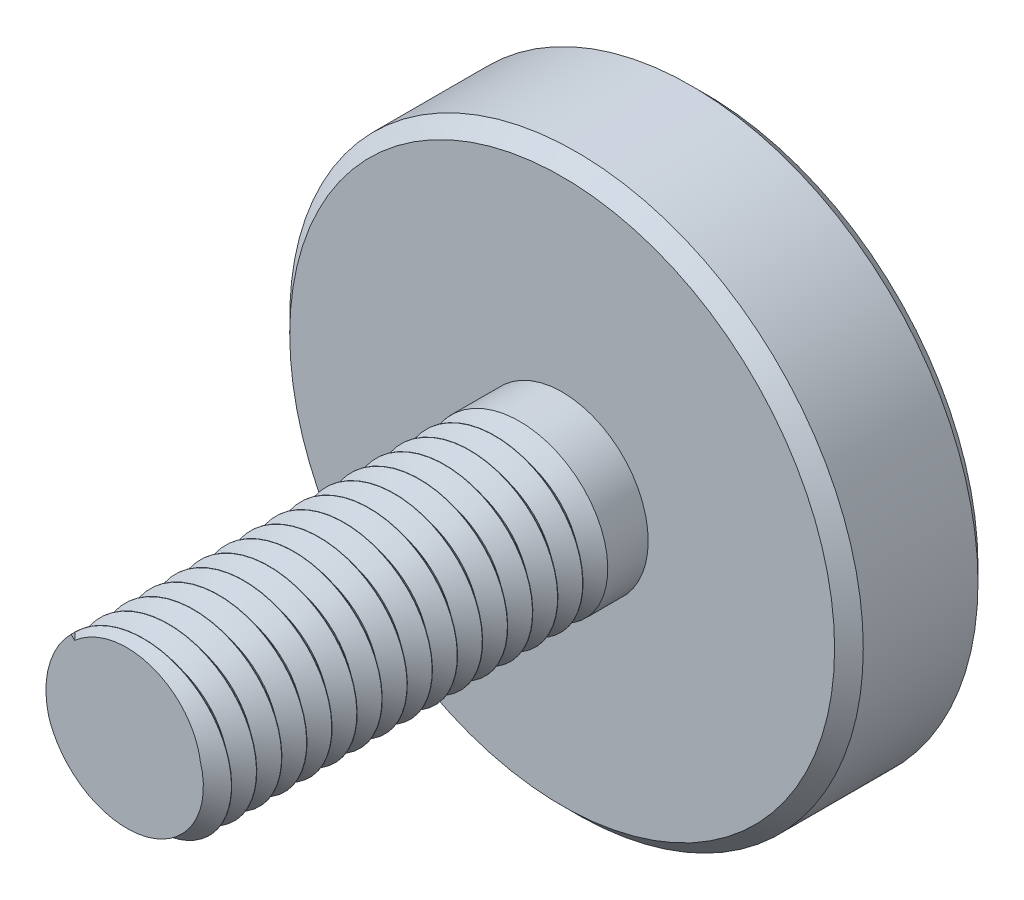
from build123d import *

# Parameters (mm, degrees)
SKETCH_1_R          = 20
EXTRUDE_1_DEPTH     = 10
SKETCH_2_R          = 6
EXTRUDE_3_DEPTH     = 30
SWEEP_1_PITCH       = 1.75
SWEEP_1_HEIGHT      = 28
SWEEP_1_RADIUS      = 6
SWEEP_1_START_ANGLE = 45
CHAMFER_1_SIZE      = 1


with BuildPart() as part:
    # 草图1 → 凸台-拉伸1 (new body)
    with BuildSketch(Plane.XY):
        Circle(SKETCH_1_R)
    extrude(amount=EXTRUDE_1_DEPTH)

    # 草图2 → 凸台-拉伸3 (add)
    with BuildSketch(Plane.XY.offset(10)):
        Circle(SKETCH_2_R)
    extrude(amount=EXTRUDE_3_DEPTH)

    # 切除-扫描1: sweep along a helix
    with BuildLine() as sweep_1_path:
        add(Helix(SWEEP_1_PITCH, SWEEP_1_HEIGHT, SWEEP_1_RADIUS, center=(0, 0, 40), direction=(0, 0, -1), mode=Mode.PRIVATE).rotate(Axis((0, 0, 40), (0, 0, -1)), SWEEP_1_START_ANGLE))
    # 草图5 → 切除-扫描1 (sweep, cut)
    with BuildSketch(Plane(origin=(0, 0, 0), x_dir=(0, 0, -1), z_dir=(1, 0, 0))):
        Polygon((-39.598251524, 6.141374382), (-37.652469247, 6.141374382), (-38.625360385, 4.883734618), align=None)
    sweep(path=sweep_1_path.line, is_frenet=True, mode=Mode.SUBTRACT)

    # 倒角1
    chamfer_1_edges = [part.edges().sort_by_distance(p)[0] for p in [
        (-20, 0, 0),
        (-20, 0, 10),
    ]]
    chamfer(chamfer_1_edges, length=CHAMFER_1_SIZE)


solid = part.part
